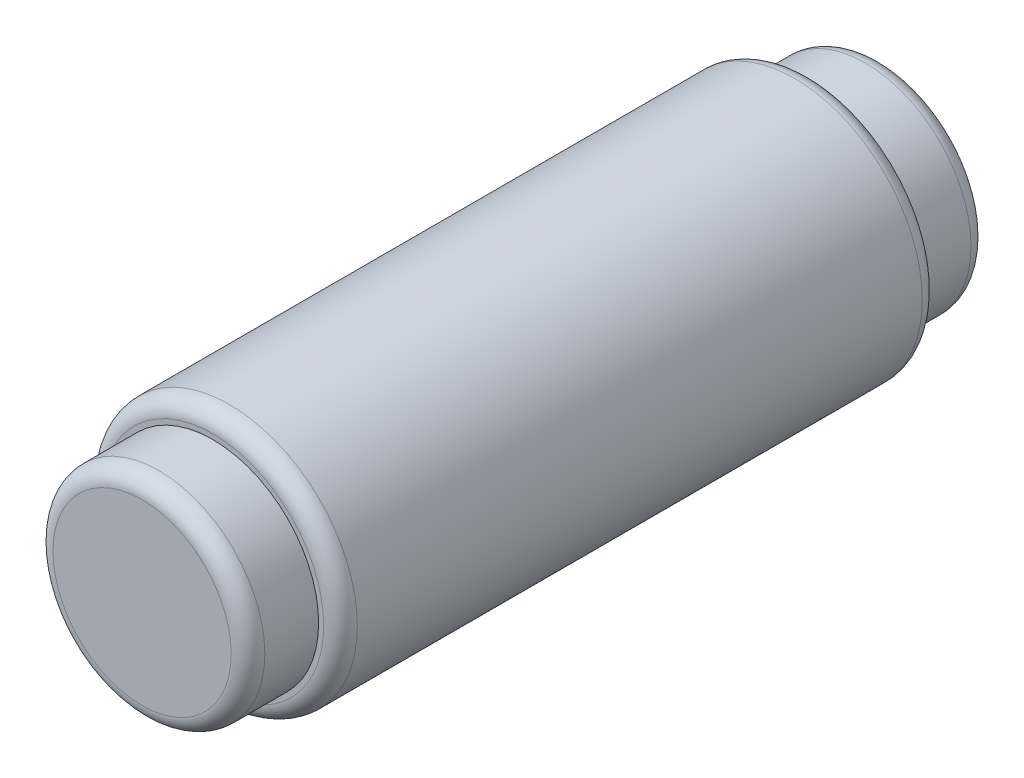
from build123d import *

# Parameters (mm, degrees)
SKETCH_1_R          = 38
EXTRUDE_1_DEPTH     = 110
SKETCH_4_OUTSIDE_W  = 126.97
SKETCH_4_OUTSIDE_H  = 126.97
SKETCH_4_OUTSIDE_R  = 31.5
CUT_EXTRUDE_1_DEPTH = 21
SKETCH_5_OUTSIDE_W  = 126.97
SKETCH_5_OUTSIDE_H  = 126.97
SKETCH_5_OUTSIDE_R  = 31.5
CUT_EXTRUDE_2_DEPTH = 21
FILLET_1_R          = 5
SKETCH_2_R          = 5.478928785
SKETCH_2_R_2        = 5.511284945
EXTRUDE_2_DEPTH     = 2


with BuildPart() as part:
    # 草图1 → 凸台-拉伸1 (new, symmetric)
    with BuildSketch(Plane.XY):
        Circle(SKETCH_1_R)
    extrude(amount=EXTRUDE_1_DEPTH, both=True)

    # 草图4 outside → 切除-拉伸1 (cut)
    with BuildSketch(Plane.XY.offset(110)):
        Rectangle(SKETCH_4_OUTSIDE_W, SKETCH_4_OUTSIDE_H)
        Circle(SKETCH_4_OUTSIDE_R, mode=Mode.SUBTRACT)
    extrude(amount=-CUT_EXTRUDE_1_DEPTH, mode=Mode.SUBTRACT)

    # 草图5 outside → 切除-拉伸2 (cut)
    with BuildSketch(Plane(origin=(0, 0, -110), x_dir=(-1, 0, 0), z_dir=(0, 0, -1))):
        Rectangle(SKETCH_5_OUTSIDE_W, SKETCH_5_OUTSIDE_H)
        with Locations(Location((0, 0, 0), (0, 0, 180))):
            Circle(SKETCH_5_OUTSIDE_R, mode=Mode.SUBTRACT)
    extrude(amount=-CUT_EXTRUDE_2_DEPTH, mode=Mode.SUBTRACT)

    # 圆角1
    fillet_1_edges = [part.edges().sort_by_distance(p)[0] for p in [
        (-31.5, 0, 110),
        (-38, 0, -89),
        (-31.5, 0, -110),
        (-38, 0, 89),
    ]]
    fillet(fillet_1_edges, radius=FILLET_1_R)

    # 草图2 → 凸台-拉伸2 (add)
    with BuildSketch(Plane(origin=(0, 0, -110), x_dir=(-1, 0, 0), z_dir=(0, 0, -1))):
        with Locations(Location((0, 15.014240139, 0), (0, 0, 180))):
            Circle(SKETCH_2_R)
        with Locations(Location((0, -16.315898799, 0), (0, 0, 180))):
            Circle(SKETCH_2_R_2)
    extrude(amount=EXTRUDE_2_DEPTH)


solid = part.part
